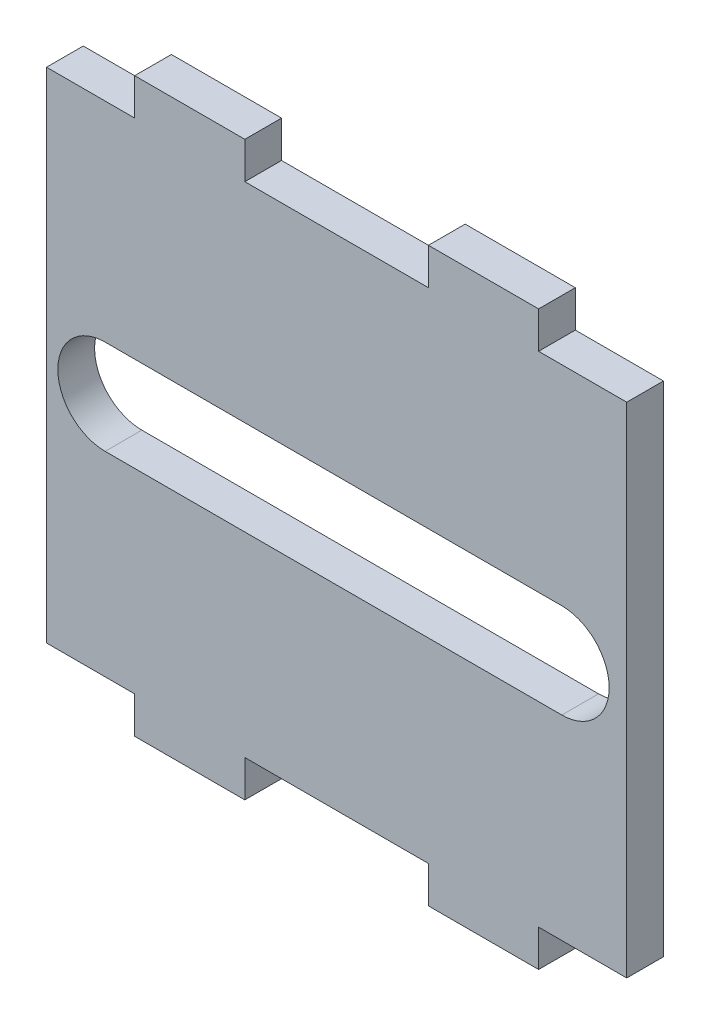
SolidWorks part; units mm, degrees
ref_plane "前视基准面" through (0, 0, 0) normal (0, 0, 1) x (1, 0, 0)
ref_plane "上视基准面" through (0, 0, 0) normal (0, 1, 0) x (1, 0, 0)
ref_plane "右视基准面" through (0, 0, 0) normal (1, 0, 0) x (0, 0, -1)
sketch "草图1" plane through (0, 0, 0) normal (0, 0, 1) x (1, 0, 0)
  line L0 (39.5, 0) -> (39.5, 90) construction
  line L1 (12, 0) -> (27, 0)
  line L2 (0, 5) -> (0, 72.9)
  line L3 (12, 77.9) -> (27, 77.9)
  line L4 (79, 5) -> (79, 72.9)
  line L5 (52, 0) -> (67, 0)
  line L6 (52, 0) -> (52, 5)
  line L8 (67, 0) -> (67, 5)
  line L10 (27, 0) -> (27, 5)
  line L12 (12, 0) -> (12, 5)
  line L14 (12, 77.9) -> (12, 72.9)
  line L16 (27, 77.9) -> (27, 72.9)
  line L17 (52, 77.9) -> (67, 77.9)
  line L18 (52, 77.9) -> (52, 72.9)
  line L20 (67, 77.9) -> (67, 72.9)
  line L21 (0, 5) -> (12, 5)
  line L22 (79, 72.9) -> (67, 72.9)
  line L25 (27, 5) -> (52, 5)
  line L26 (67, 5) -> (79, 5)
  line L27 (52, 72.9) -> (27, 72.9)
  line L28 (12, 72.9) -> (0, 72.9)
  dimension "D1" = 77.9
  dimension "D3" = 5
  dimension "D4" = 15
  dimension "D5" = 25
  dimension "D6" = 25
extrude "凸台-拉伸1" add sketch "草图1" along normal blind 5
sketch "草图2" plane through (0, 0, 0) normal (0, 0, -1) x (-1, 0, 0)
  line L0 (-70.1631, 38.0313) -> (-7.9796, 38.0313) construction
  line L1 (-70.1631, 44.471) -> (-7.9796, 44.471)
  line L2 (-70.1631, 31.5916) -> (-7.9796, 31.5916)
  arc A0 (-70.1631, 44.471) -> (-70.1631, 31.5916) centre (-70.1631, 38.0313) ccw
  arc A1 (-7.9796, 31.5916) -> (-7.9796, 44.471) centre (-7.9796, 38.0313) ccw
  point P2 (-39.0714, 38.0313)
extrude "切除-拉伸2" cut sketch "草图2" against normal blind 5
